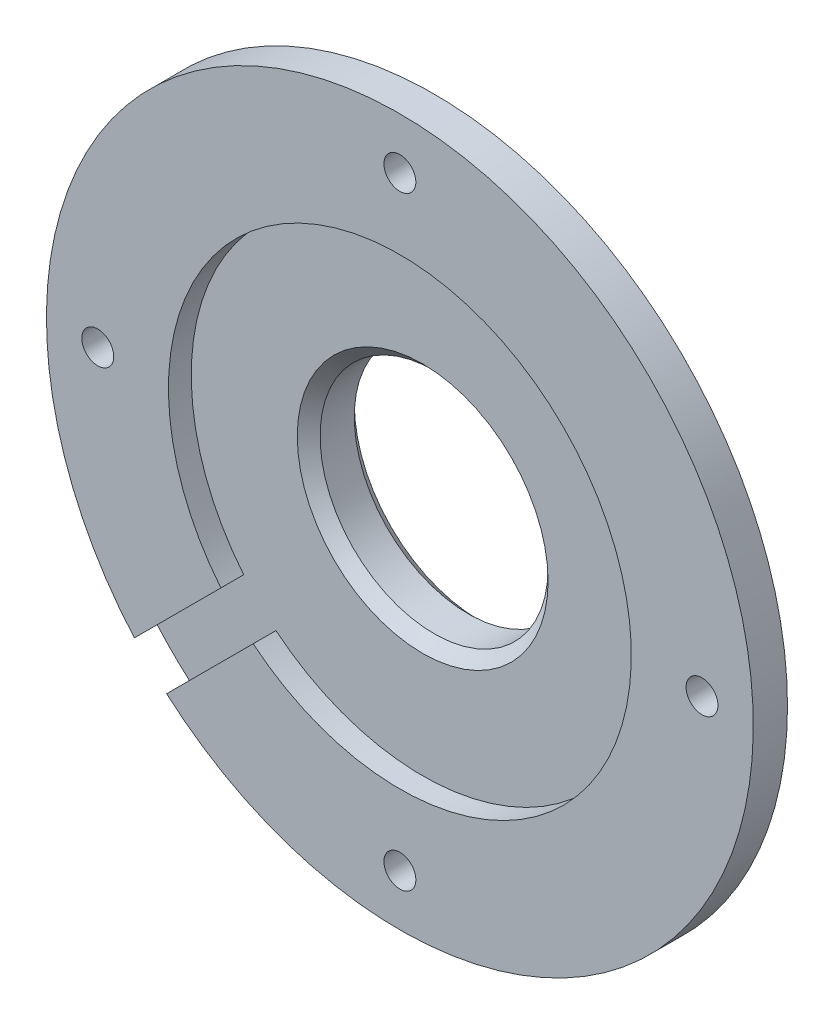
from build123d import *

# Parameters (mm, degrees)
SKETCH1_R           = 12
BOSS_EXTRUDE1_DEPTH = 2
SKETCH2_R           = 15.5
SKETCH2_R_2         = 0.7
BOSS_EXTRUDE2_DEPTH = 1.5
SKETCH3_R           = 10.15
CUT_EXTRUDE1_DEPTH  = 1
FILLET1_R           = 1.2
SKETCH4_R           = 1.25
CUT_EXTRUDE2_DEPTH  = 0.5
SKETCH5_R           = 5
CUT_EXTRUDE3_DEPTH  = 23.19797288
CHAMFER1_SIZE       = 0.5
CUT_EXTRUDE4_DEPTH  = 1


with BuildPart() as part:
    # Sketch1 → Boss-Extrude1 (new body)
    with BuildSketch(Plane.XY):
        Circle(SKETCH1_R)
    extrude(amount=BOSS_EXTRUDE1_DEPTH)

    # Sketch2 → Boss-Extrude2 (add)
    with BuildSketch(Plane.XY.offset(2)):
        Circle(SKETCH2_R)
        with Locations((0, 13.25)):
            Circle(SKETCH2_R_2, mode=Mode.SUBTRACT)
        with Locations((13.25, 0)):
            Circle(SKETCH2_R_2, mode=Mode.SUBTRACT)
        with Locations((0, -13.25)):
            Circle(SKETCH2_R_2, mode=Mode.SUBTRACT)
        with Locations((-13.25, 0)):
            Circle(SKETCH2_R_2, mode=Mode.SUBTRACT)
    extrude(amount=BOSS_EXTRUDE2_DEPTH)

    # Sketch3 → Cut-Extrude1 (cut)
    with BuildSketch(Plane.XY.offset(3.5)):
        Circle(SKETCH3_R)
    extrude(amount=-CUT_EXTRUDE1_DEPTH, mode=Mode.SUBTRACT)

    # Fillet1
    fillet1_edges = [part.edges().sort_by_distance(p)[0] for p in [
        (-12, 0, 0),
    ]]
    fillet(fillet1_edges, radius=FILLET1_R)

    # Sketch4 → Cut-Extrude2 (cut)
    with BuildSketch(Plane(origin=(0, 0, 2), x_dir=(-1, 0, 0), z_dir=(0, 0, -1))):
        with Locations((0, 13.25)):
            Circle(SKETCH4_R)
        with Locations((13.25, 0)):
            Circle(SKETCH4_R)
        with Locations((0, -13.25)):
            Circle(SKETCH4_R)
        with Locations((-13.25, 0)):
            Circle(SKETCH4_R)
    extrude(amount=-CUT_EXTRUDE2_DEPTH, mode=Mode.SUBTRACT)

    # Sketch5 → Cut-Extrude3 (cut, through all)
    with BuildSketch(Plane(origin=(0, 0, 0), x_dir=(-1, 0, 0), z_dir=(0, 0, -1))):
        Circle(SKETCH5_R)
    extrude(amount=-CUT_EXTRUDE3_DEPTH, mode=Mode.SUBTRACT)

    # Chamfer1
    chamfer1_edges = [part.edges().sort_by_distance(p)[0] for p in [
        (5, 0, 2.5),
        (5, 0, 0),
    ]]
    chamfer(chamfer1_edges, length=CHAMFER1_SIZE)

    # Sketch6 → Cut-Extrude4 (cut)
    with BuildSketch(Plane.XY.offset(3.5)):
        Polygon((-0.707106781, 0.707106781), (0.707106781, -0.707106781), (-10.253048327, -11.66726189), (-11.66726189, -10.253048327), align=None)
    extrude(amount=-CUT_EXTRUDE4_DEPTH, mode=Mode.SUBTRACT)


solid = part.part
